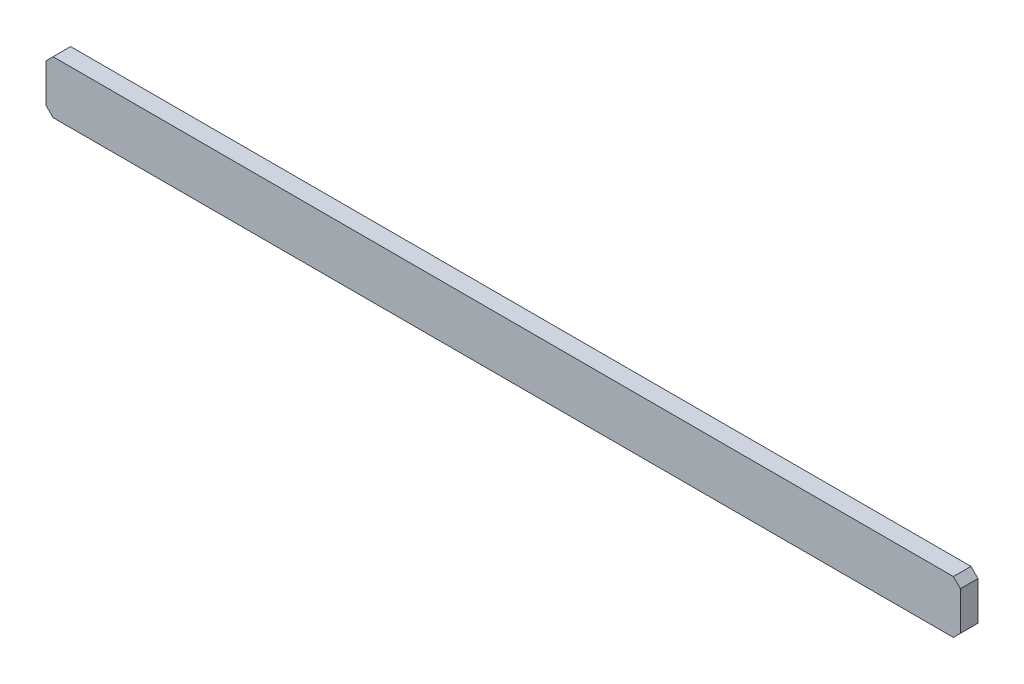
from build123d import *

# Parameters (mm, degrees)
SKETCH_1_W      = 260
SKETCH_1_H      = 15
EXTRUDE_1_DEPTH = 5
CHAMFER_1_SIZE  = 2


with BuildPart() as part:
    # 草图1 → 凸台-拉伸1 (new body)
    with BuildSketch(Plane.XY):
        Rectangle(SKETCH_1_W, SKETCH_1_H)
    extrude(amount=EXTRUDE_1_DEPTH)

    # 倒角1
    chamfer_1_edges = [part.edges().sort_by_distance(p)[0] for p in [
        (130, -7.5, 2.5),
        (-130, -7.5, 2.5),
        (-130, 7.5, 2.5),
        (130, 7.5, 2.5),
    ]]
    chamfer(chamfer_1_edges, length=CHAMFER_1_SIZE)


solid = part.part
